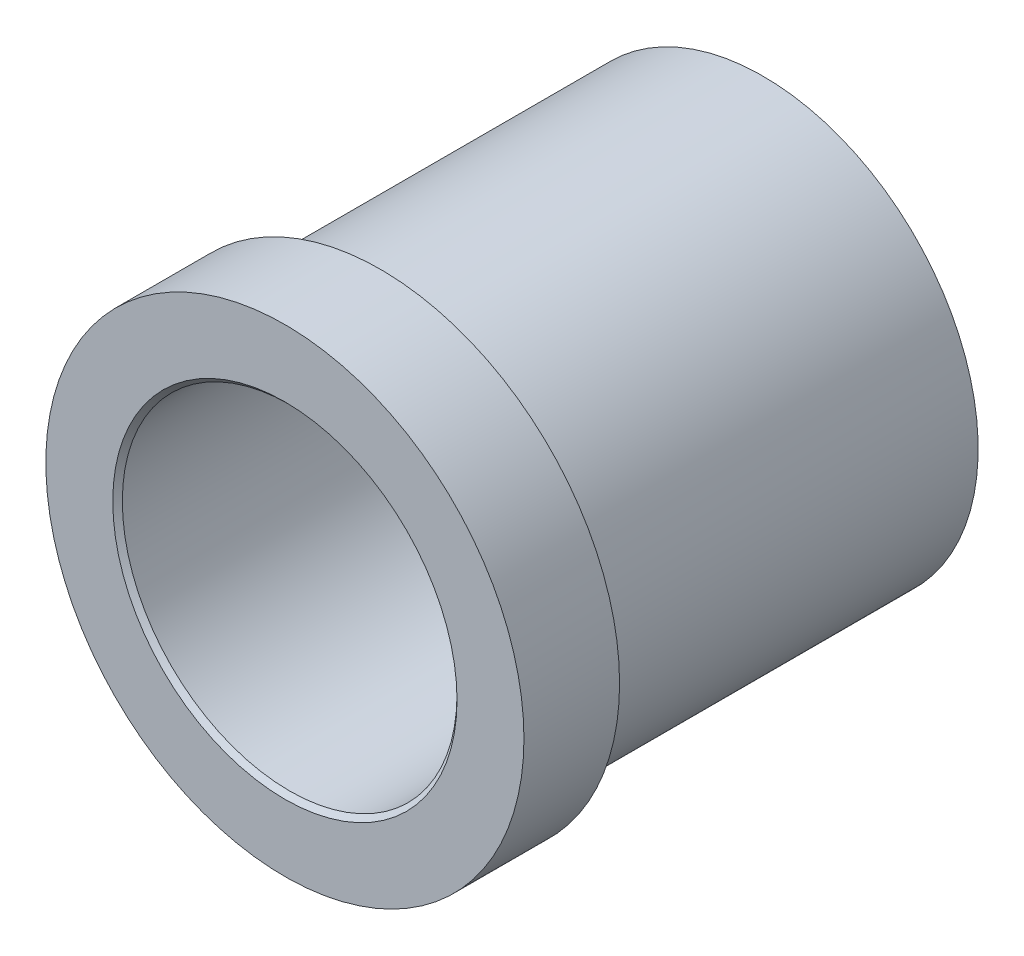
from build123d import *

# Parameters (mm, degrees)
SKETCH_1_R          = 25
EXTRUDE_1_DEPTH     = 10
SKETCH_2_R          = 22.5
EXTRUDE_2_DEPTH     = 40
SKETCH_3_R          = 17.5
CUT_EXTRUDE_1_DEPTH = 80
CHAMFER_1_SIZE      = 0.5


with BuildPart() as part:
    # 草图1 → 凸台-拉伸1 (new body)
    with BuildSketch(Plane.XY):
        Circle(SKETCH_1_R)
    extrude(amount=EXTRUDE_1_DEPTH)

    # 草图2 → 凸台-拉伸2 (add)
    with BuildSketch(Plane(origin=(0, 0, 0), x_dir=(-1, 0, 0), z_dir=(0, 0, -1))):
        Circle(SKETCH_2_R)
    extrude(amount=EXTRUDE_2_DEPTH)

    # 草图3 → 切除-拉伸1 (cut)
    with BuildSketch(Plane(origin=(0, 0, -40), x_dir=(-1, 0, 0), z_dir=(0, 0, -1))):
        Circle(SKETCH_3_R)
    extrude(amount=-CUT_EXTRUDE_1_DEPTH, mode=Mode.SUBTRACT)

    # 倒角1
    chamfer_1_edges = [part.edges().sort_by_distance(p)[0] for p in [
        (17.5, 0, 10),
    ]]
    chamfer(chamfer_1_edges, length=CHAMFER_1_SIZE)


solid = part.part
